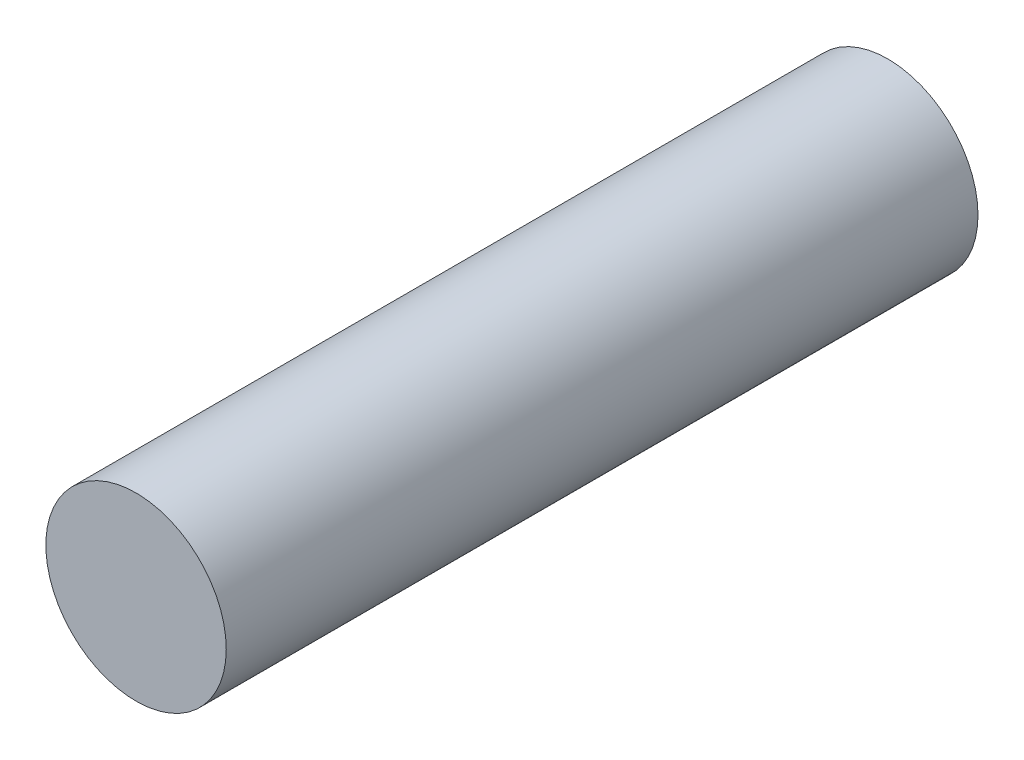
from build123d import *

# Parameters (mm, degrees)
SKETCH1_R           = 12
BOSS_EXTRUDE1_DEPTH = 100


with BuildPart() as part:
    # Sketch1 → Boss-Extrude1 (new body)
    with BuildSketch(Plane.XY):
        Circle(SKETCH1_R)
    extrude(amount=BOSS_EXTRUDE1_DEPTH)


solid = part.part
